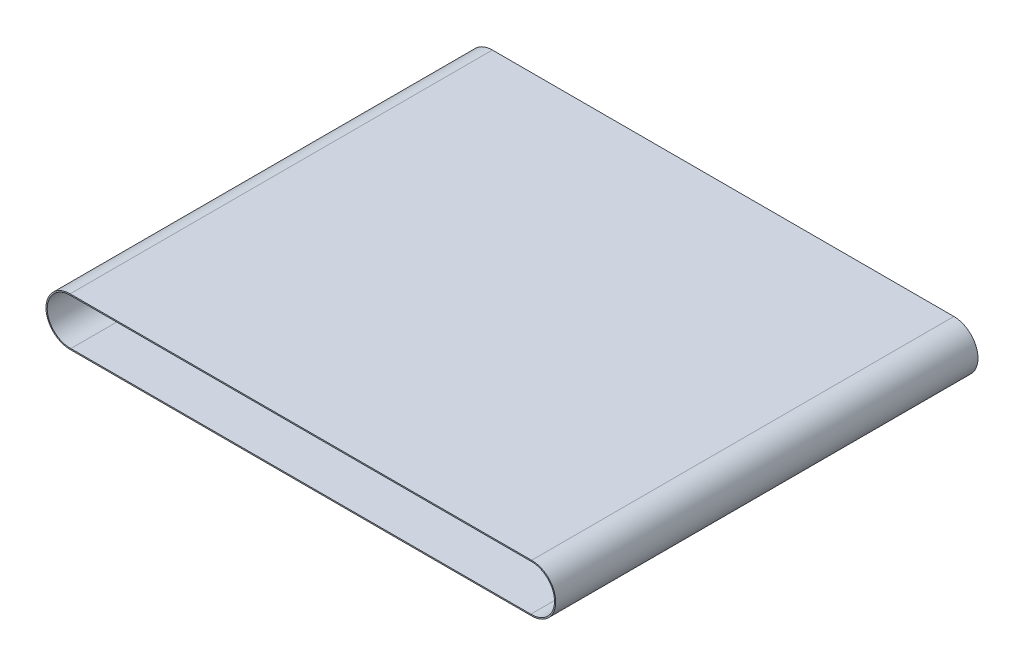
from build123d import *

# Parameters (mm, degrees)
EXTRUDE_1_DEPTH      = 350
EXTRUDE_2_DEPTH      = 352
EXTRUDE_2_DEPTH_BACK = 361


with BuildPart() as part:
    # 草图1 → 拉伸-薄壁1 (new, symmetric)
    with BuildSketch(Plane.XY):
        with BuildLine():
            Line((381.234257801, -39.979968693), (-381.234257801, -39.979968693))
            ThreePointArc((-381.234257801, -39.979968693), (-422.49499186, -0.632950347), (-382.5, 40))
            Line((-382.5, 40), (382.5, 40))
            ThreePointArc((382.5, 40), (422.49499186, -0.632950347), (381.234257801, -39.979968693))
        make_face()
        with BuildLine():
            Line((381.26631524, -37.979968693), (-381.26631524, -37.979968693))
            ThreePointArc((-381.26631524, -37.979968693), (-420.494991843, -0.616923686), (-382.5, 38))
            Line((-382.5, 38), (382.5, 38))
            ThreePointArc((382.5, 38), (420.494991843, -0.616923686), (381.26631524, -37.979968693))
        make_face(mode=Mode.SUBTRACT)
    extrude(amount=EXTRUDE_1_DEPTH, both=True)

    # 草图4 → 凸台-拉伸2 (add, two sides: drawn at the far end of the back side and taken through both)
    with BuildSketch(Plane(origin=(0, 0, 0), x_dir=(0, 0, -1), z_dir=(1, 0, 0)).offset(-EXTRUDE_2_DEPTH_BACK)):
        Polygon((4, 38), (-4, 38), (-2.5, 33), (2.5, 33), align=None)
    extrude(amount=EXTRUDE_2_DEPTH + EXTRUDE_2_DEPTH_BACK)


solid = part.part
